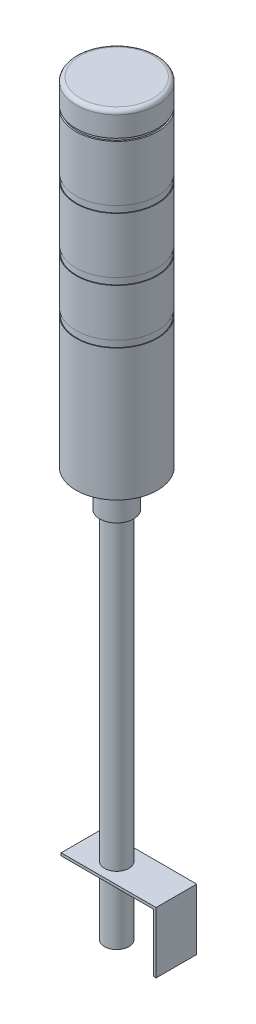
SolidWorks part; units mm, degrees
ref_plane "前基準面" through (0, 0, 0) normal (0, 0, 1) x (1, 0, 0)
ref_plane "上基準面" through (0, 0, 0) normal (0, 1, 0) x (1, 0, 0)
ref_plane "右基準面" through (0, 0, 0) normal (1, 0, 0) x (0, 0, -1)
sketch "草图1" plane through (0, 0, 0) normal (0, 0, 1) x (1, 0, 0)
  line L0 (0, 0) -> (0, 202.5)
  line L1 (30, 232.5) -> (182.5, 232.5)
  line L2 (212.5, 262.5) -> (212.5, 698.5)
  arc A0 (0, 202.5) -> (30, 232.5) centre (30, 202.5) cw
  arc A1 (182.5, 232.5) -> (212.5, 262.5) centre (182.5, 262.5) ccw
  point P7 (0, 232.5)
  point P10 (212.5, 232.5)
  dimension "D4" = 30
  dimension "D1" = 232.5
  dimension "D2" = 212.5
  dimension "D3" = 466
sketch "草图2" plane through (0, 0, 0) normal (0, 1, 0) x (1, 0, 0)
  circle A0 centre (0, 0) radius 24
  dimension "D1" = 48
sweep "扫描4" add profiles "草图2" path "草图1"
shell "抽壳1" thickness 5
sketch "草图4" plane through (0, 698.5, 0) normal (0, 1, 0) x (-1, 0, 0)
  circle A0 centre (-212.5, 0) radius 60
  dimension "D1" = 120
extrude "拉伸1" add sketch "草图4" along normal blind 6
sketch "草图5" plane through (0, 704.5, 0) normal (0, 1, 0) x (-1, 0, 0)
  line L1 (-312.5, -125) -> (-112.5, -125)
  line L2 (-312.5, -125) -> (-312.5, 125)
  line L3 (-312.5, 125) -> (-112.5, 125)
  line L4 (-112.5, -125) -> (-112.5, 125)
  circle A0 centre (-212.5, 0) radius 60 construction
  dimension "D4" = 125
  dimension "D1" = 250
  dimension "D2" = 200
  dimension "D3" = 100
extrude "拉伸2" add sketch "草图5" along normal blind 280
sketch "草图6" plane through (0, 984.5, 0) normal (0, 1, 0) x (-1, 0, 0)
  line L0 (-312.5, 125) -> (-312.5, -125) construction
  line L1 (-312.5, -125) -> (-112.5, -125) construction
  circle A0 centre (-212.5, -75) radius 30
  dimension "D3" = 60
  dimension "D1" = 100
  dimension "D2" = 50
extrude "拉伸3" add sketch "草图6" along normal blind 97.1
sketch "草图7" plane through (0, 1081.6, 0) normal (0, 1, 0) x (-1, 0, 0)
  circle A0 centre (-212.5, -75) radius 29.5
  dimension "D1" = 59
extrude "拉伸4" add sketch "草图7" along normal blind 5
sketch "草图8" plane through (0, 1086.6, 0) normal (0, 1, 0) x (-1, 0, 0)
  circle A0 centre (-212.5, -75) radius 30 construction
  circle A1 centre (-212.5, -75) radius 30
extrude "拉伸5" add sketch "草图8" along normal blind 35
sketch "草图9" plane through (0, 1121.6, 0) normal (0, 1, 0) x (-1, 0, 0)
  circle A0 centre (-212.5, -75) radius 29.5 construction
  circle A1 centre (-212.5, -75) radius 29.5
extrude "拉伸6" add sketch "草图9" along normal blind 5
sketch "草图10" plane through (0, 1126.6, 0) normal (0, 1, 0) x (-1, 0, 0)
  circle A0 centre (-212.5, -75) radius 30 construction
  circle A1 centre (-212.5, -75) radius 30
extrude "拉伸7" add sketch "草图10" along normal blind 41
sketch "草图11" plane through (0, 1167.6, 0) normal (0, 1, 0) x (-1, 0, 0)
  circle A0 centre (-212.5, -75) radius 29.5 construction
  circle A1 centre (-212.5, -75) radius 29.5
extrude "拉伸8" add sketch "草图11" along normal blind 5
sketch "草图12" plane through (0, 1172.6, 0) normal (0, 1, 0) x (-1, 0, 0)
  circle A0 centre (-212.5, -75) radius 30 construction
  circle A1 centre (-212.5, -75) radius 30
extrude "拉伸9" add sketch "草图12" along normal blind 41
sketch "草图13" plane through (0, 1213.6, 0) normal (0, 1, 0) x (-1, 0, 0)
  circle A0 centre (-212.5, -75) radius 29
  dimension "D1" = 58
extrude "拉伸10" add sketch "草图13" along normal blind 2
sketch "草图14" plane through (0, 1215.6, 0) normal (0, 1, 0) x (-1, 0, 0)
  circle A0 centre (-212.5, -75) radius 30
  dimension "D1" = 60
extrude "拉伸11" add sketch "草图14" along normal blind 18
fillet "圆角1" radius 3 1 edges at (212.5, 1233.6, -45)
sketch "草图15" plane through (0, 0, 0) normal (0, -1, 0) x (1, 0, 0)
  circle A0 centre (0, 0) radius 22.5
  dimension "D1" = 45
extrude "切除-拉伸1" cut sketch "草图15" against normal blind 26 flip side to cut
sketch "草图16" plane through (312.5, 0, 0) normal (1, 0, 0) x (0, 0, -1)
  line L1 (125, 984.5) -> (-875.9505, 984.5)
  line L2 (125, 984.5) -> (125, -388.0462)
  line L3 (125, -388.0462) -> (-875.9505, -388.0462)
  line L4 (-875.9505, 984.5) -> (-875.9505, -388.0462)
extrude "拉伸12" cut sketch "草图16" against normal through all
sketch "草图17" plane through (0, 984.5, 0) normal (0, -1, 0) x (1, 0, 0)
  circle A0 centre (212.5, -75) radius 12.5
  dimension "D1" = 25
extrude "拉伸13" add sketch "草图17" along normal blind 27
sketch "草图24" plane through (0, 957.5, 0) normal (0, -1, 0) x (1, 0, 0)
  circle A0 centre (212.5, -75) radius 9
  dimension "D1" = 18
extrude "凸台-拉伸1" add sketch "草图24" along normal blind 275
ref_plane "基准面1" through (0, 682.5, 0) normal (0, -1, 0) x (1, 0, 0)
ref_plane "基准面2" through (0, 0, -75) normal (0, 0, 1) x (1, 0, 0)
sketch "草图26" plane through (0, 0, -75) normal (0, 0, 1) x (1, 0, 0)
  line L0 (186.5, 732.5) -> (256.5, 732.5)
  line L1 (256.5, 732.5) -> (256.5, 687.5)
  line L2 (203.5, 682.5) -> (221.5, 682.5) construction
  line L3 (221.5, 682.5) -> (221.5, 957.5) construction
  dimension "D1" = 70
  dimension "D2" = 50
  dimension "D3" = 45
  dimension "D4" = 35
extrude "拉伸-薄壁1" add sketch "草图26" along normal mid plane 30 thin
